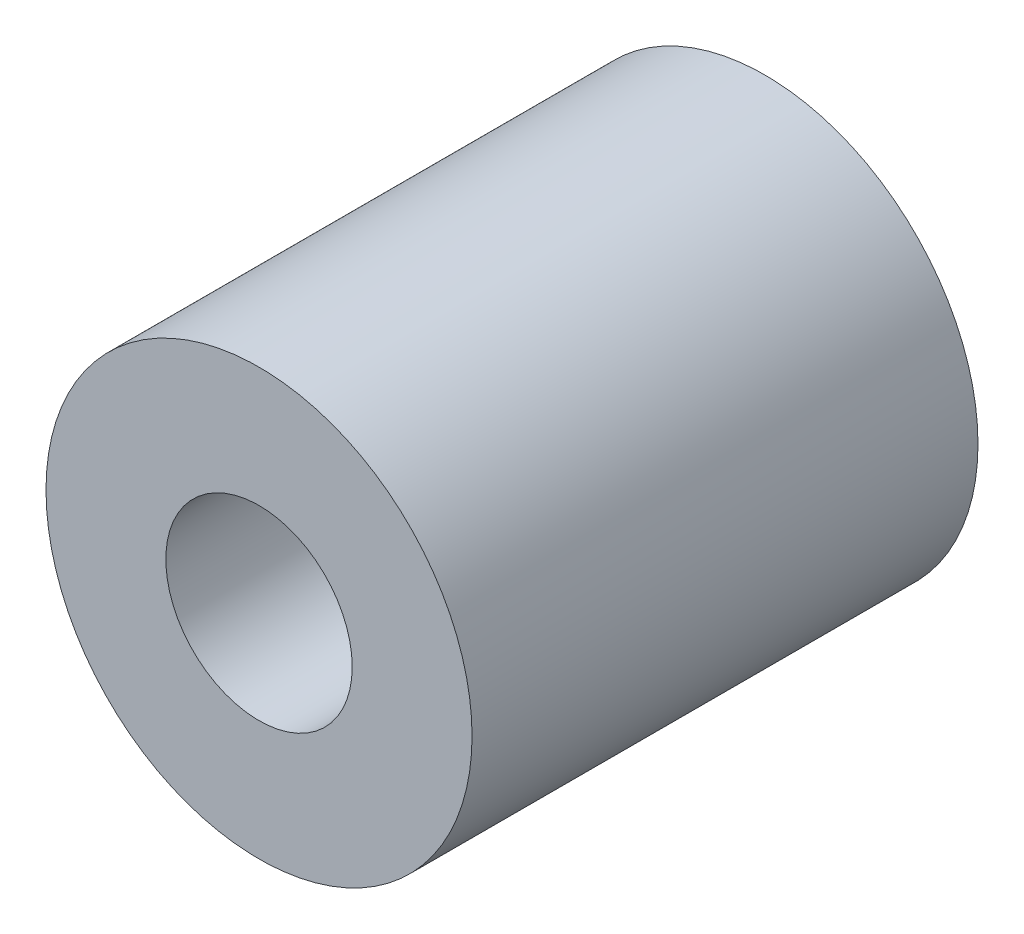
from build123d import *

# Parameters (mm, degrees)
SKETCH1_R           = 16
BOSS_EXTRUDE1_DEPTH = 38
M16_TAPPED_HOLE1_D  = 14


with BuildPart() as part:
    # Sketch1 → Boss-Extrude1 (new body)
    with BuildSketch(Plane.XY):
        Circle(SKETCH1_R)
    extrude(amount=BOSS_EXTRUDE1_DEPTH)

    # M16 Tapped Hole1 (through all)
    with Locations(Plane.XY.offset(38)):
        with Locations((0, 0)):
            Hole(M16_TAPPED_HOLE1_D / 2)


solid = part.part
